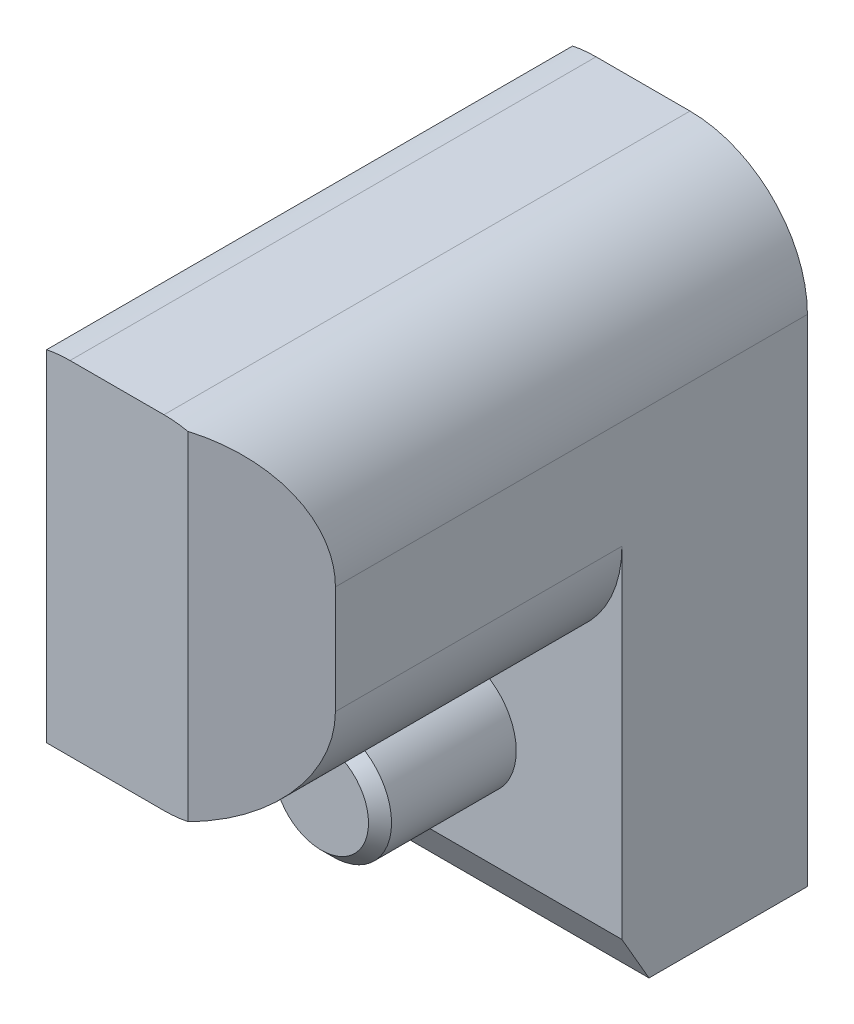
from build123d import *

# Parameters (mm, degrees)
BOSS_EXTRUDE1_DEPTH     = 22.4
CUT_EXTRUDE1_DEPTH      = 7
CUT_EXTRUDE1_DEPTH_BACK = 7
CUT_EXTRUDE2_DEPTH      = 19.8
CUT_EXTRUDE3_DEPTH      = 2.5
CUT_EXTRUDE4_DEPTH      = 5.925
CUT_EXTRUDE4_DEPTH_BACK = 5.925
CUT_EXTRUDE5_DEPTH      = 7
CUT_EXTRUDE5_DEPTH_BACK = 7
CUT_EXTRUDE6_DEPTH      = 26.1
CUT_EXTRUDE6_DEPTH_BACK = 26.1


with BuildPart() as part:
    # Sketch1 → Boss-Extrude1 (new body)
    with BuildSketch(Plane.XY):
        with BuildLine():
            Line((-7, 21.1), (-7, 0))
            Line((-7, 0), (7, 0))
            Line((7, 0), (7, 21.1))
            ThreePointArc((7, 21.1), (5.535533906, 24.635533906), (2, 26.1))
            Line((2, 26.1), (-2, 26.1))
            ThreePointArc((-2, 26.1), (-5.535533906, 24.635533906), (-7, 21.1))
        make_face()
    extrude(amount=BOSS_EXTRUDE1_DEPTH)

    # Sketch2 → Cut-Extrude1 (cut, two sides: drawn at the far end of the back side and taken through both)
    with BuildSketch(Plane(origin=(0, 0, 0), x_dir=(0, 0, -1), z_dir=(1, 0, 0)).offset(-CUT_EXTRUDE1_DEPTH_BACK)):
        Polygon((-7.9, 2), (-7.9, 0), (-6.745299462, 0), align=None)
    extrude(amount=CUT_EXTRUDE1_DEPTH + CUT_EXTRUDE1_DEPTH_BACK, mode=Mode.SUBTRACT)

    # Sketch4 → Cut-Extrude2 (cut)
    with BuildSketch(Plane.XY.offset(7.9)):
        with BuildLine():
            Line((-7, 26.1), (-7, 0))
            Line((-7, 0), (9, 0))
            Line((9, 0), (9, 16.5))
            Line((9, 16.5), (7, 16.5))
            ThreePointArc((7, 16.5), (5.535533906, 12.964466094), (2, 11.5))
            Line((2, 11.5), (-3, 11.5))
            Line((-3, 11.5), (-3, 26.1))
            Line((-3, 26.1), (-7, 26.1))
        make_face()
    extrude(amount=CUT_EXTRUDE2_DEPTH, mode=Mode.SUBTRACT)

    # Sketch3 → Cut-Revolve1 (revolve, cut)
    with BuildSketch(Plane(origin=(0, 0, 0), x_dir=(0, 0, -1), z_dir=(1, 0, 0)), mode=Mode.PRIVATE) as cut_revolve1_sk:
        Polygon((-0.7, 6.7), (-0.7, 10.45), (-1.2, 10.95), (-5.7, 10.95), (-5.7, 11.7), (0, 11.7), (0, 6.7), align=None)
    revolve(cut_revolve1_sk.sketch.rotate(Axis((0, 6.7, 0), (0, 0, 1)), 270), axis=Axis((0, 6.7, 0), (0, 0, 1)), mode=Mode.SUBTRACT)

    # Sketch5 → Cut-Extrude3 (cut)
    with BuildSketch(Plane(origin=(0, 0, 0.7), x_dir=(-1, 0, 0), z_dir=(0, 0, -1))):
        Polygon((1.154700538, 4.7), (2.309401077, 6.7), (1.154700538, 8.7), (-1.154700538, 8.7), (-2.309401077, 6.7), (-1.154700538, 4.7), align=None)
    extrude(amount=-CUT_EXTRUDE3_DEPTH, mode=Mode.SUBTRACT)

    # Sketch6 → Cut-Extrude4 (cut, two sides: drawn at the far end of the back side and taken through both)
    with BuildSketch(Plane.XY.offset(5.925).offset(-CUT_EXTRUDE4_DEPTH_BACK)):
        with BuildLine():
            Line((-7, 14.2), (-5, 14.2))
            ThreePointArc((-5, 14.2), (-3.585786438, 14.785786438), (-3, 16.2))
            Line((-3, 16.2), (-3, 26.1))
            Line((-3, 26.1), (-7, 26.1))
            Line((-7, 26.1), (-7, 14.2))
        make_face()
    extrude(amount=CUT_EXTRUDE4_DEPTH + CUT_EXTRUDE4_DEPTH_BACK, mode=Mode.SUBTRACT)

    # Sketch7 → Cut-Extrude5 (cut, two sides: drawn at the far end of the back side and taken through both)
    with BuildSketch(Plane(origin=(0, 0, 0), x_dir=(0, 0, -1), z_dir=(1, 0, 0)).offset(-CUT_EXTRUDE5_DEPTH_BACK)):
        with BuildLine():
            Line((-11.419615242, 11.4), (-7.9, 11.4))
            Line((-7.9, 11.4), (-7.9, 11.7))
            ThreePointArc((-7.9, 11.7), (-8.4, 12.566025404), (-9.4, 12.566025404))
            Line((-9.4, 12.566025404), (-11.419615242, 11.4))
        make_face()
    extrude(amount=CUT_EXTRUDE5_DEPTH + CUT_EXTRUDE5_DEPTH_BACK, mode=Mode.SUBTRACT)

    # Sketch8 → Cut-Extrude6 (cut, two sides: drawn at the far end of the back side and taken through both)
    with BuildSketch(Plane(origin=(0, 0, 0), x_dir=(1, 0, 0), z_dir=(0, 1, 0)).offset(-CUT_EXTRUDE6_DEPTH_BACK)):
        Polygon((3.016283143, -22.4), (7, -22.4), (7, -20.1), align=None)
    extrude(amount=CUT_EXTRUDE6_DEPTH + CUT_EXTRUDE6_DEPTH_BACK, mode=Mode.SUBTRACT)

    # Sketch9 → Revolve1 (revolve)
    with BuildSketch(Plane(origin=(0, 0, 0), x_dir=(0, 0, -1), z_dir=(1, 0, 0)), mode=Mode.PRIVATE) as revolve1_sk:
        Polygon((-13.7, 6.7), (-13.7, 8.7095), (-13.2095, 9.2), (-7.9, 9.2), (-7.9, 6.7), align=None)
    revolve(revolve1_sk.sketch.rotate(Axis((0, 6.7, 7.9), (0, 0, 1)), 270), axis=Axis((0, 6.7, 7.9), (0, 0, 1)))


solid = part.part
